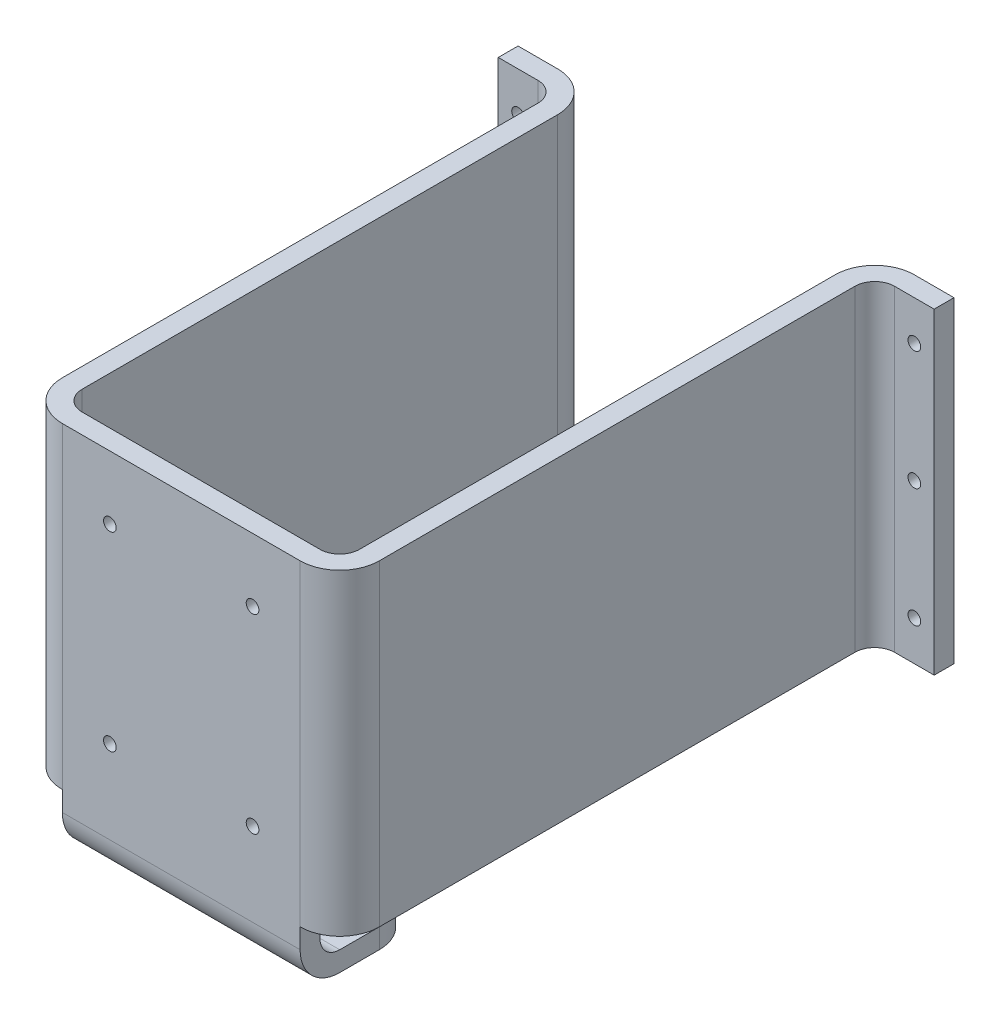
SolidWorks part; units mm, degrees
ref_plane "Front Plane" through (0, 0, 0) normal (0, 0, 1) x (1, 0, 0)
ref_plane "Top Plane" through (0, 0, 0) normal (0, 1, 0) x (1, 0, 0)
ref_plane "Right Plane" through (0, 0, 0) normal (1, 0, 0) x (0, 0, -1)
sketch "Sketch1" plane through (0, 0, 0) normal (0, 1, 0) x (1, 0, 0)
  line L2 (0, 0) -> (0, 134.3061)
  line L3 (0, 134.3061) -> (5, 134.3061)
  line L4 (5, -0.6939) -> (5, 134.3061)
  line L5 (5, -0.6939) -> (75, -0.6939)
  line L6 (0, 0) -> (0, -5.6939)
  line L7 (0, -5.6939) -> (35.8571, -5.6939)
  line L9 (35.8571, -5.6939) -> (80, -5.6939)
  line L10 (75, -0.6939) -> (75, 134.3061)
  line L11 (75, 134.3061) -> (80, 134.3061)
  line L12 (80, -5.6939) -> (80, 134.3061)
  dimension "D1" = 5
  dimension "D2" = 5
  dimension "D3" = 5
  dimension "D4" = 140
  dimension "D5" = 140
  dimension "D6" = 80
extrude "Boss-Extrude1" add sketch "Sketch1" along normal blind 80
sketch "Sketch2" plane through (80, 0, 0) normal (1, 0, 0) x (0, 0, -1)
  line L0 (-5.6939, 80) -> (134.3061, 80) construction
  line L1 (134.3061, 0) -> (129.3061, 0)
  line L2 (134.3061, 0) -> (134.3061, 80)
  line L3 (134.3061, 80) -> (129.3061, 80)
  line L4 (129.3061, 0) -> (129.3061, 80)
  dimension "D1" = 5
extrude "Boss-Extrude2" add sketch "Sketch2" along normal blind 15
sketch "Sketch3" plane through (0, 0, 0) normal (-1, 0, 0) x (0, 0, 1)
  line L0 (-134.3061, 80) -> (5.6939, 80) construction
  line L1 (-134.3061, 0) -> (-129.3061, 0)
  line L2 (-134.3061, 0) -> (-134.3061, 80)
  line L3 (-134.3061, 80) -> (-129.3061, 80)
  line L4 (-129.3061, 0) -> (-129.3061, 80)
  dimension "D1" = 5
extrude "Boss-Extrude3" add sketch "Sketch3" along normal blind 15
fillet "Fillet1" radius 10 4 edges at (75, 40, -134.3061) (5, 40, -134.3061) (80, 40, 5.6939) (0, 40, 5.6939)
fillet "Fillet2" radius 5 4 edges at (80, 40, -129.3061) (0, 40, -129.3061) (5, 40, 0.6939) (75, 40, 0.6939)
sketch "Sketch4" plane through (0, 0, 0) normal (0, -1, 0) x (1, 0, 0)
  line L0 (10, 5.6939) -> (70, 5.6939) construction
  line L1 (10, 5.6939) -> (70, 5.6939)
  line L2 (10, 5.6939) -> (10, 0.6939)
  line L3 (10, 0.6939) -> (70, 0.6939)
  line L4 (70, 5.6939) -> (70, 0.6939)
  point P6 (10, 3.1939)
  dimension "D1" = 5
  dimension "D2" = 60
  dimension "D3" = 0
extrude "Boss-Extrude4" add sketch "Sketch4" along normal blind 15
sketch "Sketch5" plane through (0, 0, 0.6939) normal (0, 0, -1) x (-1, 0, 0)
  line L0 (-70, -15) -> (-70, 0) construction
  line L1 (-70, -10) -> (-10, -10)
  line L2 (-70, -10) -> (-70, -15)
  line L3 (-70, -15) -> (-10, -15)
  line L4 (-10, -10) -> (-10, -15)
  dimension "D1" = 5
extrude "Boss-Extrude5" add sketch "Sketch5" along normal blind 25
fillet "Fillet3" radius 5 1 edges at (40, -10, 0.6939)
fillet "Fillet4" radius 10 1 edges at (40, -15, 5.6939)
sketch "Sketch6" plane through (0, -15, 0) normal (0, -1, 0) x (1, 0, 0)
  line L0 (70, -24.3061) -> (10, -24.3061) construction
  circle A0 centre (17.5, -16.3061) radius 1.6
  circle A1 centre (62.5, -16.3061) radius 1.6
  point P6 (40, -24.3061)
  dimension "D1" = 45
  dimension "D2" = 3.2
  dimension "D3" = 8
  dimension "D4" = 22.5
extrude "Cut-Extrude1" cut sketch "Sketch6" against normal blind 10
fillet "Fillet5" radius 10 2 edges at (70, -12.5, -24.3061) (10, -12.5, -24.3061)
sketch "Sketch7" plane through (0, 0, 5.6939) normal (0, 0, 1) x (1, 0, 0)
  line L0 (10, 80) -> (70, 80) construction
  line L1 (22, 64) -> (58, 64) construction
  line L2 (22, 64) -> (22, 16) construction
  line L3 (22, 16) -> (58, 16) construction
  line L4 (58, 64) -> (58, 16) construction
  line L6 (70, 0) -> (70, 80) construction
  circle A0 centre (22, 64) radius 1.6
  circle A1 centre (58, 64) radius 1.6
  circle A2 centre (58, 16) radius 1.6
  circle A3 centre (22, 16) radius 1.6
  dimension "D5" = 3.2
  dimension "D6" = 3.2
  dimension "D7" = 3.2
  dimension "D8" = 3.2
  dimension "D1" = 36
  dimension "D2" = 48
  dimension "D3" = 16
  dimension "D4" = 12
extrude "Cut-Extrude2" cut sketch "Sketch7" against normal through all
sketch "Sketch8" plane through (0, 0, -129.3061) normal (0, 0, 1) x (1, 0, 0)
  line L0 (95, 80) -> (95, 0) construction
  line L2 (-5, 0) -> (-5, 80) construction
  circle A0 centre (-10, 70) radius 1.6
  circle A1 centre (-10, 40) radius 1.6
  circle A2 centre (-10, 10) radius 1.6
  circle A3 centre (90, 70) radius 1.6
  circle A4 centre (90, 40) radius 1.6
  circle A5 centre (90, 10) radius 1.6
  point P18 (-5, 40)
  dimension "D1" = 3.2
  dimension "D2" = 100
  dimension "D3" = 5
  dimension "D4" = 60
  dimension "D5" = 60
  dimension "D6" = 30
  dimension "D7" = 30
  dimension "D8" = 0
extrude "Cut-Extrude3" cut sketch "Sketch8" against normal through all
